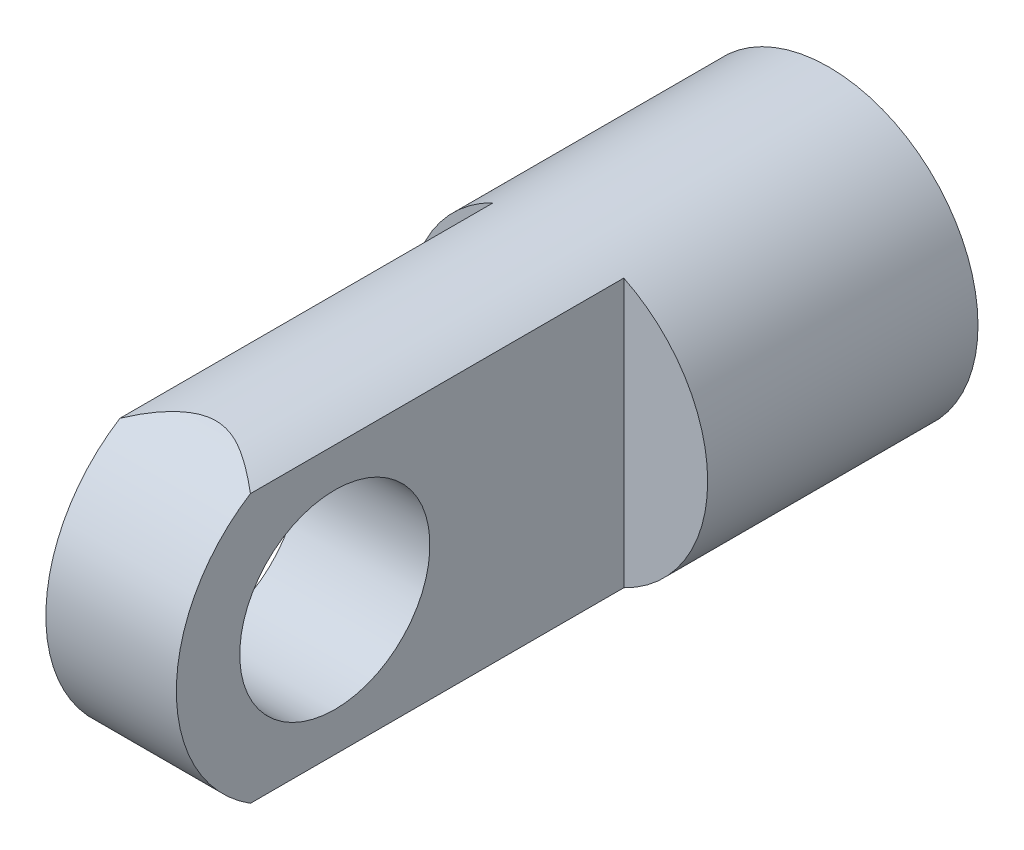
from build123d import *

# Parameters (mm, degrees)
SKETCH_1_R             = 8
EXTRUDE_1_DEPTH        = 38.5
SKETCH_2_W             = 5
SKETCH_2_H             = 16
CUT_EXTRUDE_1_DEPTH    = 24
SKETCH_3_R             = 5.1
CUT_EXTRUDE_2_DEPTH    = 24
CUT_EXTRUDE_3_DEPTH    = 41.969500851
HOLE_WIZARD_M8_1_D     = 6.8
HOLE_WIZARD_M8_1_DEPTH = 12
HOLE_WIZARD_M8_1_TIP   = 2.042926105


with BuildPart() as part:
    # 草图1 → 凸台-拉伸1 (new body)
    with BuildSketch(Plane.XY):
        Circle(SKETCH_1_R)
    extrude(amount=EXTRUDE_1_DEPTH)

    # 草图2 → 切除-拉伸1 (cut)
    with BuildSketch(Plane.XY.offset(38.5)):
        with Locations((6, 0)):
            Rectangle(SKETCH_2_W, SKETCH_2_H)
        with Locations((-6, 0)):
            Rectangle(SKETCH_2_W, SKETCH_2_H)
    extrude(amount=-CUT_EXTRUDE_1_DEPTH, mode=Mode.SUBTRACT)

    # 草图3 → 切除-拉伸2 (cut)
    with BuildSketch(Plane(origin=(3.5, 0, 0), x_dir=(0, 0, -1), z_dir=(1, 0, 0))):
        with Locations(Location((-30, 0, 0), (0, 0, 90))):
            Circle(SKETCH_3_R)
    extrude(amount=-CUT_EXTRUDE_2_DEPTH, mode=Mode.SUBTRACT)

    # 草图4 → 切除-拉伸3 (cut, through all)
    with BuildSketch(Plane(origin=(3.5, 0, 0), x_dir=(0, 0, -1), z_dir=(1, 0, 0))):
        with BuildLine():
            Line((-30, 8.5), (-30, 11))
            Line((-30, 11), (-45, 11))
            Line((-45, 11), (-45, -11))
            Line((-45, -11), (-30, -11))
            Line((-30, -11), (-30, -8.5))
            ThreePointArc((-30, -8.5), (-38.5, 0), (-30, 8.5))
        make_face()
    extrude(amount=-CUT_EXTRUDE_3_DEPTH, mode=Mode.SUBTRACT)

    # M8 螺纹孔1
    with Locations(Plane(origin=(0, 0, 0), x_dir=(-1, 0, 0), z_dir=(0, 0, -1))):
        with Locations((0, 0)):
            Hole(HOLE_WIZARD_M8_1_D / 2, depth=HOLE_WIZARD_M8_1_DEPTH)
            with Locations((0, 0, -(HOLE_WIZARD_M8_1_DEPTH + HOLE_WIZARD_M8_1_TIP / 2))):  # 118° drill point
                Cone(0, HOLE_WIZARD_M8_1_D / 2, HOLE_WIZARD_M8_1_TIP, mode=Mode.SUBTRACT)


solid = part.part
